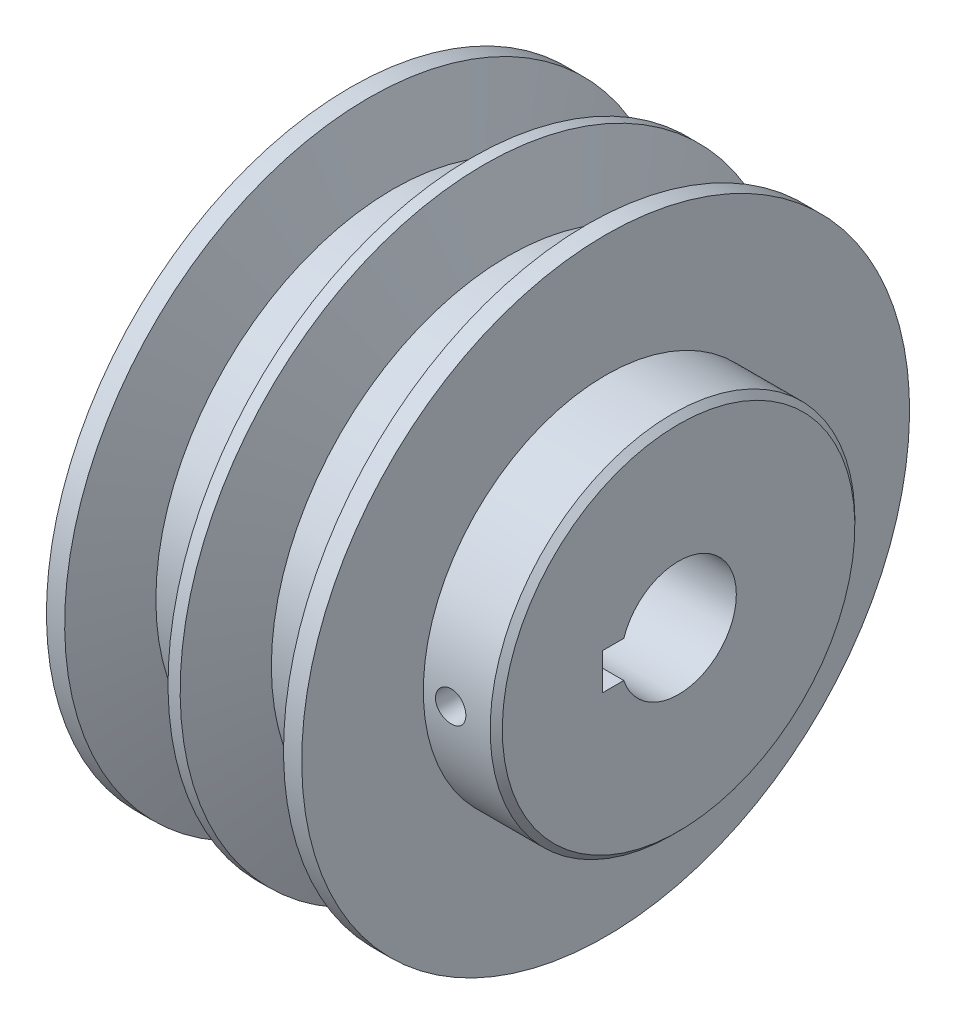
SolidWorks part; units mm, degrees
ref_plane "Front Plane" through (0, 0, 0) normal (0, 0, 1) x (1, 0, 0)
ref_plane "Top Plane" through (0, 0, 0) normal (0, 1, 0) x (1, 0, 0)
ref_plane "Right Plane" through (0, 0, 0) normal (1, 0, 0) x (0, 0, -1)
sketch "Sketch1" plane through (0, 0, 0) normal (0, 0, 1) x (1, 0, 0)
  line L0 (0, 0) -> (0, 50)
  line L1 (0, 50) -> (3, 50)
  line L2 (3, 50) -> (7.0037, 39)
  line L3 (7.0037, 39) -> (15.9963, 39)
  line L4 (15.9963, 39) -> (20, 50)
  line L5 (20, 50) -> (22, 50)
  line L6 (22, 50) -> (26.0037, 39)
  line L7 (26.0037, 39) -> (34.9963, 39)
  line L8 (34.9963, 39) -> (39, 50)
  line L9 (39, 50) -> (42, 50)
  line L10 (42, 50) -> (42, 30)
  line L11 (42, 30) -> (54, 30)
  line L12 (54, 30) -> (54, 0)
  line L13 (54, 0) -> (0, 0)
  line L14 (11.5, 52.8466) -> (11.5, 21.6016) construction
  line L15 (30.5, 54.4911) -> (30.5, 21.6016) construction
  dimension "D1" = 3
  dimension "D2" = 2
  dimension "D3" = 3
  dimension "D4" = 17
  dimension "D5" = 17
  dimension "D6" = 11
  dimension "D7" = 11
  dimension "D8" = 8.5
  dimension "D9" = 20
  dimension "D10" = 40
  dimension "D11" = 8.5
  dimension "D13" = 12
  dimension "D14" = 50
  dimension "D15" = 30
revolve "Revolve1" add sketch "Sketch1" angle 360 about L13
sketch "Sketch2" plane through (54, 0, 0) normal (1, 0, 0) x (0, 0, -1)
  circle A0 centre (0, 0) radius 9.5
  dimension "D1" = 19
extrude "Cut-Extrude1" cut sketch "Sketch2" against normal blind 70
hole_wizard "M6 Tapped Hole1" positions "Sketch6" profile "Sketch5" tap size "M6" standard "GB"
sketch "Sketch6" plane through (0, 0, 0) normal (0, 0, 1) x (1, 0, 0)
  line L0 (54, -30) -> (54, 30) construction
  point P2 (46.5, 0)
  dimension "D1" = 7.5
sketch "Sketch5" plane through (46.5, 0, 0) normal (1, 0, 0) x (0, 1, 0)
  line L0 (0, 0) -> (0, 51.5022)
  line L1 (0, 51.5022) -> (2.5, 50)
  line L2 (2.5, 50) -> (2.5, 0)
  line L5 (2.5, 0) -> (0, 0)
  line L10 (0, 51.5022) -> (-2.5, 50) construction
  line L11 (0, -6.35) -> (0, 107.95) construction
  dimension "螺纹孔钻头直径" = 5
  dimension "螺纹孔钻头深度" = 50
  dimension "导头角度" = 118
cosmetic thread "Hole thread 1" parameters "D1"=12, "D2"=6
chamfer "Chamfer1" distance 1 angle 45 1 edges at (54, 30, 0)
sketch "Sketch7" plane through (54, 0, 0) normal (1, 0, 0) x (0, 0, -1)
  line L1 (-12.5, -3) -> (-6.5, -3)
  line L2 (-12.5, -3) -> (-12.5, 3)
  line L3 (-12.5, 3) -> (-6.5, 3)
  line L4 (-6.5, -3) -> (-6.5, 3)
  line L5 (-12.5, -3) -> (-6.5, 3) construction
  line L6 (-12.5, 3) -> (-6.5, -3) construction
  circle A0 centre (0, 0) radius 9.5 construction
  point P0 (-9.5, 0)
  dimension "D1" = 6
  dimension "D2" = 6
extrude "Cut-Extrude2" cut sketch "Sketch7" against normal blind 70
